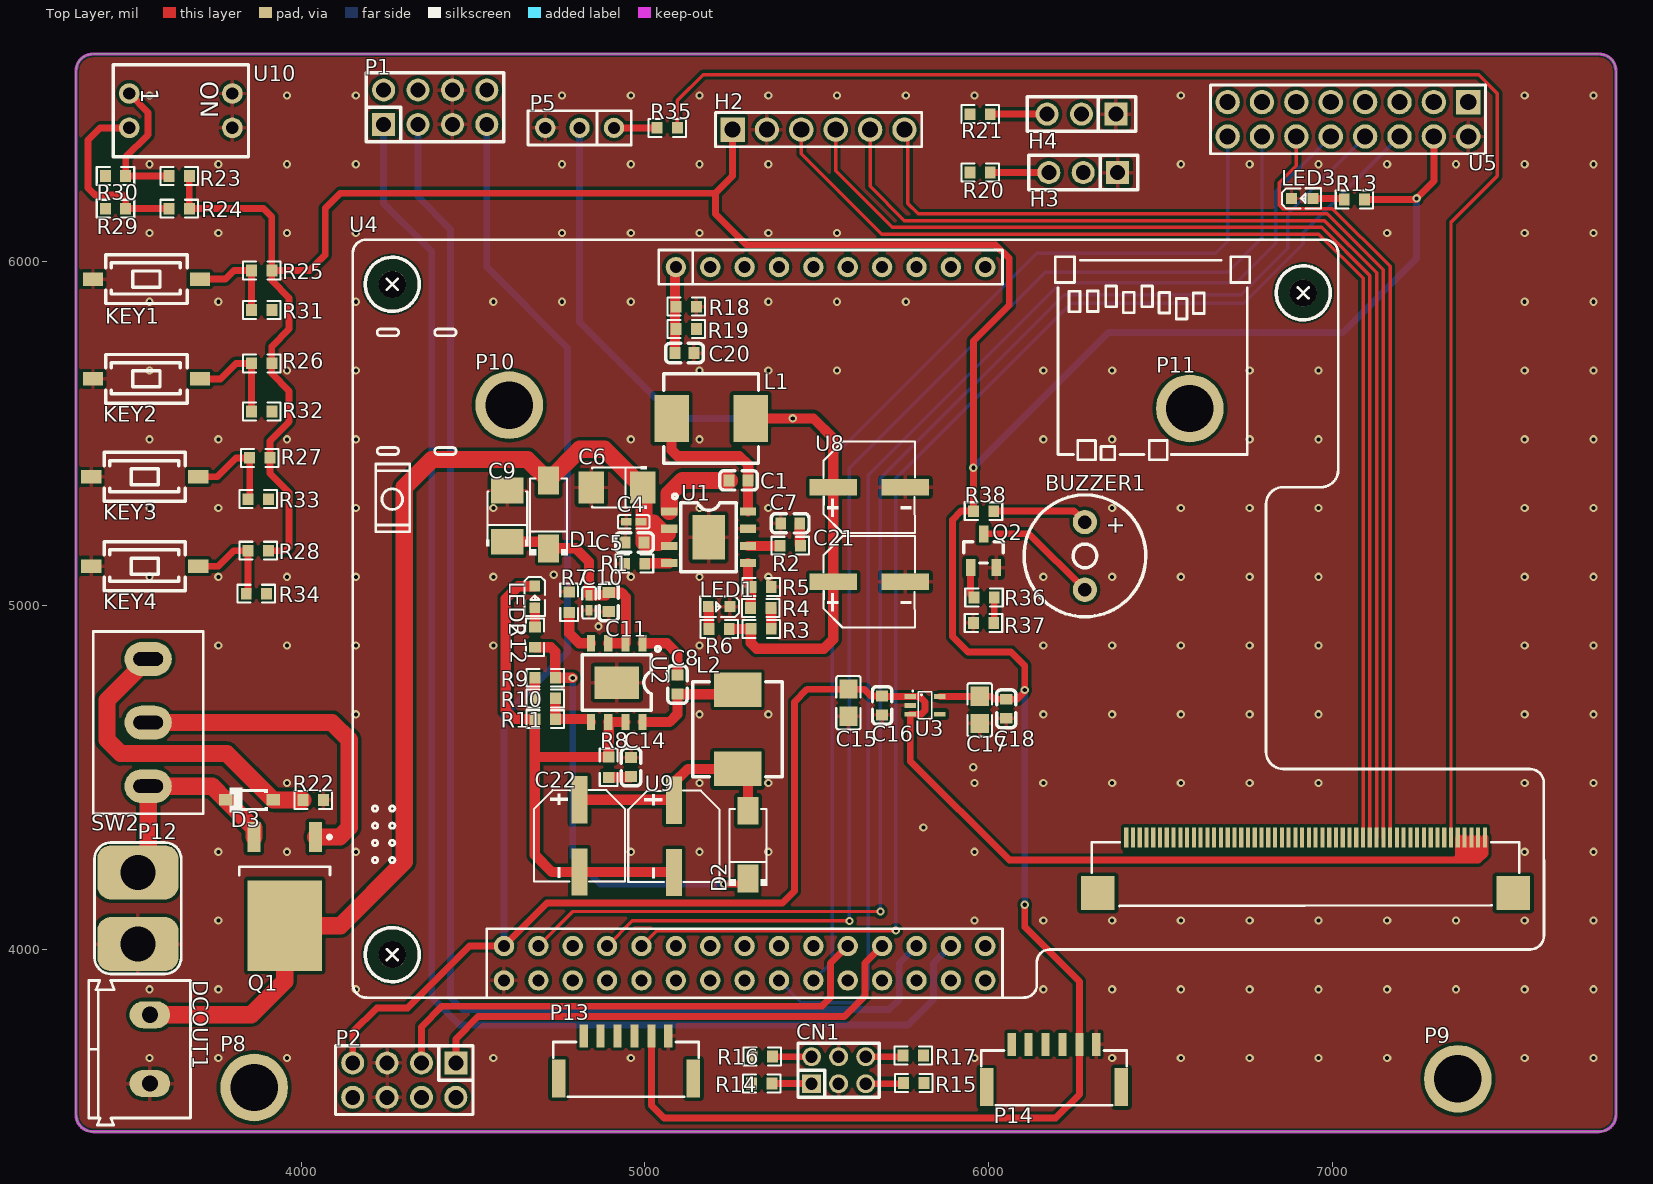
[diagram p0: Top Layer view]
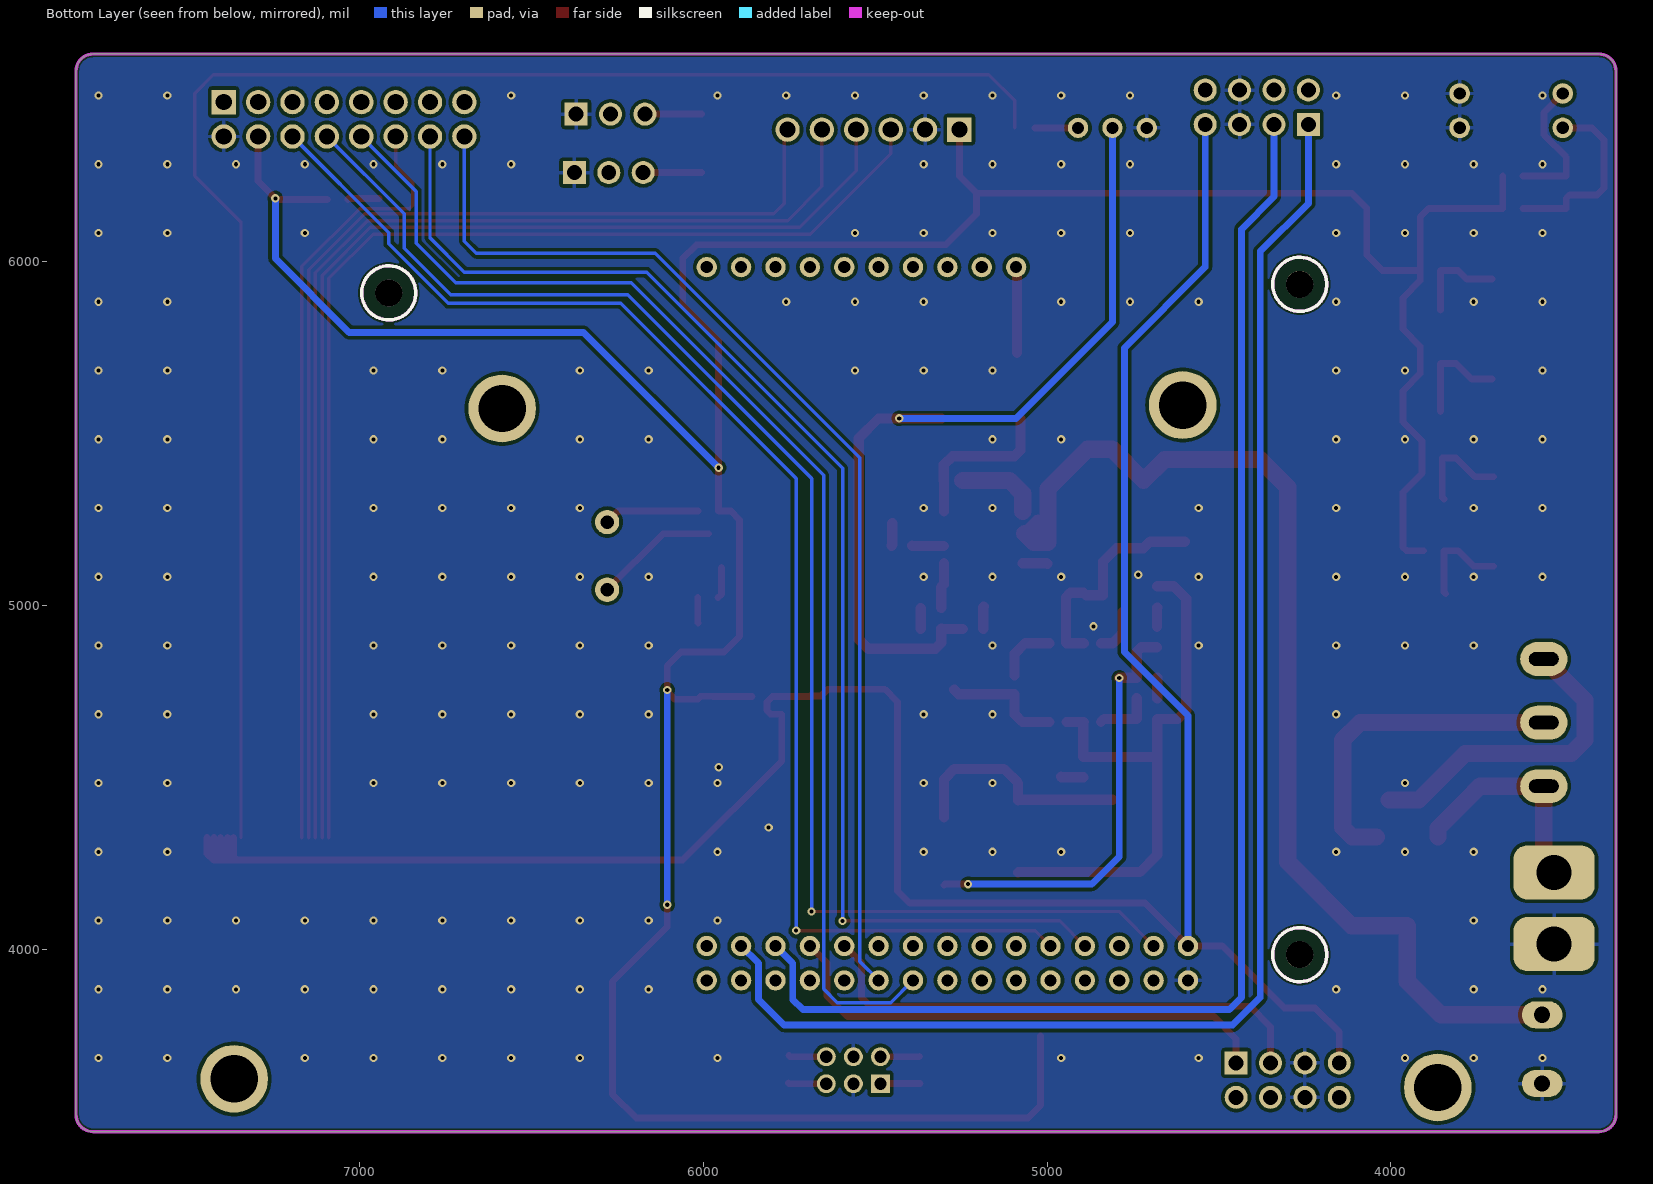
[diagram p1: Bottom Layer view, seen from below]
# Altium PCB MISC62349.pcbdoc
Units mil, origin at the board's own origin, x right, y up, seen from the top; angles counter-clockwise.
Board outline 4479.92 x 3135.04 mil, 2 copper layers (Top Layer, Bottom Layer), stack 62.206 mil thick; 94 components, 95 nets, 352 pads, 194 vias.

## Layer stack, top to bottom
Top Solder Mask Layer: solder mask 0.394, Dk 3.3
Top Layer: signal copper 1.379
Dielectric1: surface 59.449, FR4, Dk 4.5
Bottom Layer: signal copper 1.378
Bottom Solder Mask Layer: solder mask 0.394, Dk 3.3

## Board outline
3395,6605 ccw(c3395,6555) 3345,6555 3345,3519.96 ccw(c3395,3519.96) 3395,3469.96 7774.92,3469.96 ccw(c7774.92,3519.96) 7824.92,3519.96 7824.92,6555 ccw(c7774.92,6555) 7774.92,6605

## Design rules (kind name [scope] priority, off if disabled: settings)
BoardOutlineClearance copperThickness2oz_1 [All] p2 off: genericclearance=7.99 ignorepadtopadclearanceinfootprint=FALSE except(0: Arc-SplitContinuation Track-SplitContinuation SMDPad-SplitContinuation THPad-SplitContinuation Via-SplitContinuation Fill-SplitContinuation Region-SplitContinuation Poly-SplitContinuation Text-SplitContinuation Hole-SplitContinuation; 5.98: Arc-CutoutEdge Track-CutoutEdge SMDPad-CutoutEdge THPad-CutoutEdge Via-CutoutEdge Text-CutoutEdge; 6.9: Hole-OutlineEdge Hole-CutoutEdge; 10: Poly-OutlineEdge Poly-CutoutEdge; 11.81: Arc-OutlineEdge Track-OutlineEdge SMDPad-OutlineEdge THPad-OutlineEdge Via-OutlineEdge Fill-OutlineEdge Region-OutlineEdge Text-OutlineEdge Fill-CutoutEdge Region-CutoutEdge)
BoardOutlineClearance Plane_innerPlane_1 [All] p4 off: genericclearance=4.02 ignorepadtopadclearanceinfootprint=FALSE except(0: Arc-SplitContinuation Track-SplitContinuation SMDPad-SplitContinuation THPad-SplitContinuation Via-SplitContinuation Fill-SplitContinuation Region-SplitContinuation Poly-SplitContinuation Text-SplitContinuation Hole-SplitContinuation; 5.98: Arc-CutoutEdge Track-CutoutEdge SMDPad-CutoutEdge THPad-CutoutEdge Via-CutoutEdge Text-CutoutEdge; 6.9: Hole-OutlineEdge Hole-CutoutEdge; 10: Poly-OutlineEdge Poly-CutoutEdge; 11.81: Arc-OutlineEdge Track-OutlineEdge SMDPad-OutlineEdge THPad-OutlineEdge Via-OutlineEdge Fill-OutlineEdge Region-OutlineEdge Text-OutlineEdge Fill-CutoutEdge Region-CutoutEdge)
BoardOutlineClearance Copper_copperRegion_1 [All] p6 off: genericclearance=4.02 ignorepadtopadclearanceinfootprint=FALSE except(0: Arc-SplitContinuation Track-SplitContinuation SMDPad-SplitContinuation THPad-SplitContinuation Via-SplitContinuation Fill-SplitContinuation Region-SplitContinuation Poly-SplitContinuation Text-SplitContinuation Hole-SplitContinuation; 5.98: Arc-CutoutEdge Track-CutoutEdge SMDPad-CutoutEdge THPad-CutoutEdge Via-CutoutEdge Text-CutoutEdge; 6.9: Hole-OutlineEdge Hole-CutoutEdge; 10: Poly-OutlineEdge Poly-CutoutEdge; 11.81: Arc-OutlineEdge Track-OutlineEdge SMDPad-OutlineEdge THPad-OutlineEdge Via-OutlineEdge Fill-OutlineEdge Region-OutlineEdge Text-OutlineEdge Fill-CutoutEdge Region-CutoutEdge)
BoardOutlineClearance copperThickness1oz_1 [All] p8: genericclearance=4.02 ignorepadtopadclearanceinfootprint=FALSE except(0: Arc-SplitContinuation Track-SplitContinuation SMDPad-SplitContinuation THPad-SplitContinuation Via-SplitContinuation Fill-SplitContinuation Region-SplitContinuation Poly-SplitContinuation Text-SplitContinuation Hole-SplitContinuation; 5.98: Arc-CutoutEdge Track-CutoutEdge SMDPad-CutoutEdge THPad-CutoutEdge Via-CutoutEdge Text-CutoutEdge; 6.9: Hole-OutlineEdge Hole-CutoutEdge; 10: Poly-OutlineEdge Poly-CutoutEdge; 11.81: Arc-OutlineEdge Track-OutlineEdge SMDPad-OutlineEdge THPad-OutlineEdge Via-OutlineEdge Fill-OutlineEdge Region-OutlineEdge Text-OutlineEdge Fill-CutoutEdge Region-CutoutEdge)
Clearance copperThickness2oz [All] p1 off: gap=7.99 ignorepadtopadclearanceinfootprint=FALSE except(5.98: SMDPad-Track SMDPad-SMDPad THPad-Track SMDPad-THPad THPad-THPad Track-Via SMDPad-Via THPad-Via Via-Via Fill-SMDPad Region-SMDPad Fill-THPad Region-THPad Fill-Via Region-Via Fill-Fill Fill-Region Region-Region Arc-Track Arc-SMDPad Arc-THPad Arc-Via Fill-Arc Region-Arc Arc-Arc Text-Track SMDPad-Text Text-THPad Text-Via Fill-Text Region-Text Arc-Text Text-Text; 6.9: Hole-Track Hole-SMDPad Hole-THPad Hole-Via Fill-Hole Region-Hole Hole-Arc Hole-Text; 10: Poly-Track Poly-SMDPad Poly-THPad Poly-Via Poly-Fill Poly-Region Poly-Poly Poly-Arc Poly-Text Poly-Hole; 11.81: Fill-Track Region-Track)
Clearance Plane_innerPlane [All] p3 off: gap=4.02 ignorepadtopadclearanceinfootprint=FALSE except(5.98: SMDPad-Track SMDPad-SMDPad THPad-Track SMDPad-THPad THPad-THPad Track-Via SMDPad-Via THPad-Via Via-Via Fill-SMDPad Region-SMDPad Fill-THPad Region-THPad Fill-Via Region-Via Fill-Fill Fill-Region Region-Region Arc-Track Arc-SMDPad Arc-THPad Arc-Via Fill-Arc Region-Arc Arc-Arc Text-Track SMDPad-Text Text-THPad Text-Via Fill-Text Region-Text Arc-Text Text-Text; 6.9: Hole-Track Hole-SMDPad Hole-THPad Hole-Via Fill-Hole Region-Hole Hole-Arc Hole-Text; 10: Poly-Track Poly-SMDPad Poly-THPad Poly-Via Poly-Fill Poly-Region Poly-Poly Poly-Arc Poly-Text Poly-Hole; 11.81: Fill-Track Region-Track)
Clearance Copper_copperRegion [All] p5 off: gap=4.02 ignorepadtopadclearanceinfootprint=FALSE except(5.98: SMDPad-Track SMDPad-SMDPad THPad-Track SMDPad-THPad THPad-THPad Track-Via SMDPad-Via THPad-Via Via-Via Fill-SMDPad Region-SMDPad Fill-THPad Region-THPad Fill-Via Region-Via Fill-Fill Fill-Region Region-Region Arc-Track Arc-SMDPad Arc-THPad Arc-Via Fill-Arc Region-Arc Arc-Arc Text-Track SMDPad-Text Text-THPad Text-Via Fill-Text Region-Text Arc-Text Text-Text; 6.9: Hole-Track Hole-SMDPad Hole-THPad Hole-Via Fill-Hole Region-Hole Hole-Arc Hole-Text; 10: Poly-Track Poly-SMDPad Poly-THPad Poly-Via Poly-Fill Poly-Region Poly-Poly Poly-Arc Poly-Text Poly-Hole; 11.81: Fill-Track Region-Track)
Clearance copperThickness1oz [All] p7: gap=4.02 ignorepadtopadclearanceinfootprint=FALSE except(5.98: SMDPad-Track SMDPad-SMDPad THPad-Track SMDPad-THPad THPad-THPad Track-Via SMDPad-Via THPad-Via Via-Via Fill-SMDPad Region-SMDPad Fill-THPad Region-THPad Fill-Via Region-Via Fill-Fill Fill-Region Region-Region Arc-Track Arc-SMDPad Arc-THPad Arc-Via Fill-Arc Region-Arc Arc-Arc Text-Track SMDPad-Text Text-THPad Text-Via Fill-Text Region-Text Arc-Text Text-Text; 6.9: Hole-Track Hole-SMDPad Hole-THPad Hole-Via Fill-Hole Region-Hole Hole-Arc Hole-Text; 10: Poly-Track Poly-SMDPad Poly-THPad Poly-Via Poly-Fill Poly-Region Poly-Poly Poly-Arc Poly-Text Poly-Hole; 11.81: Fill-Track Region-Track)
DiffPairsRouting differentialPair [All] p1: maxlimit=6 minlimit=6 mostfreqgap=6 toplayer_minwidth=5 toplayer_prefwidth=10 toplayer_maxwidth=100 toplayer_mingap=6 toplayer_prefgap=6 toplayer_maxgap=6 bottomlayer_minwidth=5 bottomlayer_prefwidth=10 bottomlayer_maxwidth=100 bottomlayer_mingap=6 bottomlayer_prefgap=6 bottomlayer_maxgap=6 maxuncoupledlength=10
HoleToHoleClearance otherClearance [All] p1: gap=11.81 allowstackedmicrovias=TRUE
Length netLength [All] p1: minlimit=0 maxlimit=0
PasteMaskExpansion pasteMaskExpansion [All] p1: expansion=0
PlaneConnect innerPlane [All] p1: planeconnectstyle=Relief reliefexpansion=20 reliefentries=4 reliefconductorwidth=10 reliefairgap=10
PolygonConnect copperRegion [All] p1: connectstyle=Relief reliefconductorwidth=10 reliefentries=4 polygonreliefangle="90 Angle" airgapwidth=10 via.connectstyle=Relief via.reliefconductorwidth=10 via.reliefentries=4 via.polygonreliefangle="90 Angle" via.airgapwidth=10
RoutingVias viaSize [All] p1: holewidth=12.01 width=24.02 viastyle="Through Hole" minholewidth=11.81 minwidth=19.68 maxholewidth=248.03 maxwidth=393.7
SolderMaskExpansion solderMaskExpansion [IsVia] p1: expansion=-1000 istentingtop=TRUE
SolderMaskExpansion solderMaskExpansion [All] p2: expansion=2 istentingtop=FALSE
Width copperThickness2oz_2 [All] p1 off: maxlimit=100 minlimit=8 preferedwidth=10
Width copperThickness1oz_2 [All] p2: maxlimit=100 minlimit=5 preferedwidth=10

## Components (designator, comment, footprint, x,y, rotation, side; value= is the part's Value field where it differs from the comment)
BUZZER1 "BEEP" BUZ-TH_BD9-P50-D0.6-FD 6280,5145 r270 top
C1 "100nF" C0603 5272.64,5364.58 r0 top
C4 "4.7uF" C0402 4967.21,5243.92 r0 top
C5 "100nF" C0603 4969.76,5183.92 r0 top
C6 "100uF" CAP-SMD_L3.5-W2.8-R-RD 4918.66,5343.92 r0 top
C7 "4.7nF" C0603 5422.64,5239.58 r0 top
C8 "100nF" C0603 5094.67,4770.44 r270 top
C9 "100uF" CAP-SMD_L3.5-W2.8-R-RD 4599.67,5260.44 r270 top
C10 "4.7uF" C0402 4837.42,5008.58 r90 top
C11 "100nF" C0603 4894.67,5010.44 r90 top
C14 "4.7nF" C0603 4959.67,4530.56 r270 top
C15 "10uF" C0805 5592.12,4717.82 r90 top
C16 "100nF" C0603 5690,4710 r90 top
C17 "10uF" C0805 5973.94,4697.19 r90 top
C18 "100nF" C0603 6050.87,4700.26 r90 top
C20 "100nF" C0603 5115,5735 r0 top
C21 "47uF" CAP-SMD_BD6.3-L6.6-W6.6-LS7.3-FD 5652.64,5069.58 r0 top
C22 "47uF" CAP-SMD_BD6.3-L6.6-W6.6-LS7.3-FD 4809.67,4330.44 r270 top
CN1 "A2005WV-2x3P" HDR-TH_6P-P2.00-V-M-R2-C3-S2.00 5563.43,3648.78 r0 top
D1 "SS54" SMA_L4.4-W2.8-LS5.4-R-RD 4719.67,5265.44 r90 top
D2 "SS54" SMA_L4.4-W2.8-LS5.4-R-RD 5300,4305 r90 top
D3 "BZT52C16" SOD-123-L 3850,4435 r180 top
DCOUT1 "DCOUT1" "KF/WJ/DG 301-2P-5.0MM" 3560,3710 r90 top
H2 "2.54-1x6P straight pin" HDR-TH_6P-P2.54-V-M-1 5505,6385 r0 top
H3 "" HDR-TH_3P-P2.54-V-M 6275,6260 r180 top
H4 "" HDR-TH_3P-P2.54-V-M 6270,6430 r180 top
KEY1 "Tact switch 3x6x2.5mm" SW-SMD_L6.0-W3.6-LS8.0 3550,5950 r180 top
KEY2 "Tact switch 3x6x2.5mm" SW-SMD_L6.0-W3.6-LS8.0 3550,5660 r180 top
KEY3 "Tact switch 3x6x2.5mm" SW-SMD_L6.0-W3.6-LS8.0 3545,5375 r180 top
KEY4 "Tact switch 3x6x2.5mm" SW-SMD_L6.0-W3.6-LS8.0 3545,5115 r180 top
L1 "4.7uH" IND-SMD_L7.0-W6.6_VCMT063T 5192.64,5544.58 r0 top
L2 "4.7uH" IND-SMD_L7.0-W6.6_VCMT063T 5269.67,4640.44 r270 top
LED1 "LTST-C190KSKT" LED0603-RD 5215.68,4997.5 r180 top
LED2 "LTST-C190KSKT" LED0603-RD 4679.67,5025.44 r270 top
LED3 "LTST-C190KSKT" LED0603-RD 6912.38,6184.58 r0 top
P1 "Straight header 2X4P 2.54mm" HDR-TH_8P-P2.54-V-M-R2-C4-S2.54 4390,6450 r0 top
P2 "Straight header 2X4P 2.54mm" HDR-TH_8P-P2.54-V-M-R2-C4-S2.54 4300,3620 r180 top
P5 "Header-D-M 1x3P" HDR1X3-M 4910,6390 r180 top
P8 "" 定位孔 3863.38,3598.68 r0 top
P9 "" 定位孔 7364.92,3623.68 r0 top
P10 "" 定位孔 4605.36,5583.68 r0 top
P11 "" 定位孔 6585.36,5573.68 r0 top
P12 "XT60_Header" "Wired T-Header ThroughHole" 3525,4120 r0 top
P13 "GH1.25-6P" ECD-GH1.25-6P-SH 4945,3670 r0 top
P14 "GH1.25-6P" ECD-GH1.25-6P-SH 6190,3645 r0 top
Q1 "HY19P03" TO-252AA 3952.25,4198.24 r270 top
Q2 "S8050" SOT-23(SOT-23-3) 5985,5160 r0 top
R1 "200kΩ" R0603 4969.76,5122.5 r0 top
R2 "20kΩ" R0603 5422.64,5174.58 r0 top
R3 "27kΩ" R0603 5337.81,4932.59 r180 top
R4 "27kΩ" R0603 5337.13,4993.16 r0 top
R5 "7.5kΩ" R0603 5337.81,5054.58 r180 top
R6 "10K" R0603 5215.68,4932.5 r0 top
R7 "200kΩ" R0603 4779.67,5010.44 r270 top
R8 "20kΩ" R0603 4894.67,4530.44 r270 top
R9 "51kΩ" R0603 4709.67,4790.44 r0 top
R10 "1.5kΩ" R0603 4709.67,4730.44 r180 top
R11 "7.5kΩ" R0603 4710,4670 r0 top
R12 "4.7kΩ" R0603 4680.17,4908.73 r270 top
R13 "2.7kΩ" R0603 7064.07,6181.76 r180 top
R14 "100Ω" R0603 5340,3610 r0 top
R15 "100Ω" R0603 5782.17,3611.35 r180 top
R16 "100Ω" R0603 5341.71,3688.78 r180 top
R17 "100Ω" R0603 5780.45,3691.35 r0 top
R18 "20kΩ" R0603 5120,5870 r0 top
R19 "200kΩ" R0603 5120,5805 r180 top
R20 "100Ω" R0603 5975,6260 r180 top
R21 "100Ω" R0603 5975,6430 r180 top
R22 "10K" R0603 4035,4435 r180 top
R23 "4.7kΩ" R0603 3645,6250 r180 top
R24 "4.7kΩ" R0603 3645,6155 r180 top
R25 "4.7kΩ" R0603 3885,5975 r180 top
R26 "4.7kΩ" R0603 3885,5705 r180 top
R27 "4.7kΩ" R0603 3880,5430 r180 top
R28 "4.7kΩ" R0603 3875,5160 r180 top
R29 "470Ω" R0603 3460,6155 r180 top
R30 "470Ω" R0603 3460,6250 r180 top
R31 "100Ω" R0603 3885,5860 r0 top
R32 "100Ω" R0603 3885,5565 r0 top
R33 "100Ω" R0603 3875,5310 r0 top
R34 "100Ω" R0603 3870,5035 r0 top
R35 "100Ω" R0603 5065,6390 r180 top
R36 "4.7kΩ" R0603 5986.46,5023.78 r180 top
R37 "1kΩ" R0603 5985,4950 r180 top
R38 "10Ω" R0603 5985,5275 r0 top
SW2 "SS-12D10L9" MTS-10x 3555,4660 r90 top
U1 "SCT2450CQSTER" ESOP-8_L4.9-W3.9-P1.27-LS6.0-BL-EP 5185.56,5198.92 r270 top
U2 "SCT2450CQSTER" ESOP-8_L4.9-W3.9-P1.27-LS6.0-BL-EP 4918.28,4776.23 r180 top
U3 "RT9013-33GU5" SC-70-5_L2.0-W1.3-P0.65-LS2.1-BR 5815,4710 r180 top
U4 "Loongson 2K0300 development board" 龙芯2K0300久久派开发板 4265,3985 r0 top
U5 "2X8PIN2.54" HDR-TH_16P-P2.54-V-M-R2-C8-S2.54 7045,6415 r180 top
U8 "220uF" CAP-SMD_BD6.3-L6.6-W6.6-LS7.2-FD 5652.64,5344.58 r0 top
U9 "220uF" CAP-SMD_BD6.3-L6.6-W6.6-LS7.2-FD 5084.43,4328.94 r270 top
U10 "2-position DIP switch" SW-TH_4P-L9.9-W6.8-P7.62-BL 3650,6440 r270 top

## Footprints (in the part's own frame and the unit in brackets; to place one, negate y for a bottom-side part, rotate by r counter-clockwise, add the part's x,y. Pads: shape width x height; smd on the part's side, far side on the other; paste and mask are expansions set on the pad)
BUZ-TH_BD9-P50-D0.6-FD [mm]
  round 1.8 hole 1: 1(-2.5,0) 2(2.5,0)
  silkscreen extent -4.5,-4.5 4.5,4.5
C0402 [mm]
  rect 0.79x0.54 smd paste-100 mask+0.051: 1(-0.545,0) 2(0.545,0)
  silkscreen extent -1.17,-0.5 1.17,0.5
C0603 [mm]
  rect 0.8x0.9 smd: 1(-0.7,0) 2(0.7,0)
  silkscreen extent -1.39,-0.71 1.39,0.71
C0805 [mm]
  rect 1.41x1.35 smd paste-100 mask+0.051: 1(-1,0) 2(1,0)
  silkscreen extent -1.96,-0.9 1.96,0.9
CAP-SMD_BD6.3-L6.6-W6.6-LS7.2-FD [mm]
  rect 3.5x1.2 smd: 1(-2.67,0) 2(2.67,0)
  silkscreen extent -3.38,-3.38 3.38,3.38
CAP-SMD_BD6.3-L6.6-W6.6-LS7.3-FD [mm]
  rect 3.5x1.2 smd: 1(-2.67,0) 2(2.67,0)
  silkscreen extent -3.38,-3.38 3.38,3.38
CAP-SMD_L3.5-W2.8-R-RD [mm]
  rect 1.9x2.376 smd: 1(1.899,0) 2(-1.899,0)
  silkscreen extent -1.83,-1.55 2.21,1.55
ECD-GH1.25-6P-SH [mm]
  rect 1x2.8 smd: 0(-4.975,-1.15) 0(4.975,-1.15)
  rect 0.6x1.7 smd: 1(3.125,2) 2(1.875,2) 3(0.625,2) 4(-0.625,2) 5(-1.875,2) 6(-3.125,2)
  silkscreen extent -5.38,-2.5 5.38,1.55
ESOP-8_L4.9-W3.9-P1.27-LS6.0-BL-EP [mm]
  rect 0.6x1.2 smd: 1(-1.905,-2.908) 2(-0.635,-2.908) 3(0.635,-2.908) 4(1.905,-2.908) 5(1.905,2.908) 6(0.635,2.908) 7(-0.635,2.908) 8(-1.905,2.908)
  rect 3.3x2.4 smd: 9(0,0)
  silkscreen extent -3.2,-2.67 2.55,2.05
HDR1X3-M [mm]
  round 1.5 hole 0.9: 1(0,0) 2(2.54,0) 3(5.08,0)
  silkscreen extent -1.27,-1.27 6.35,1.27
HDR-TH_3P-P2.54-V-M [mm]
  rect 1.7x1.7 hole 1.1: 1(-2.54,0)
  round 1.7 hole 1.1: 2(0,0) 3(2.54,0)
  silkscreen extent -4.02,-1.27 4.02,1.27
HDR-TH_6P-P2.00-V-M-R2-C3-S2.00 [mm]
  rect 1.4x1.4 hole 0.9 paste+0 mask+0.051: 1(-2,-1)
  round 1.4 hole 0.9 paste+0 mask+0.051: 2(-2,1) 3(0,-1) 4(0,1) 5(2,-1) 6(2,1)
  silkscreen extent -3,-2 3,2
HDR-TH_6P-P2.54-V-M-1 [mm]
  rect 1.8x1.8 hole 1.2: 1(-6.35,0)
  round 1.8 hole 1.2: 2(-3.81,0) 3(-1.27,0) 4(1.27,0) 5(3.81,0) 6(6.35,0)
  silkscreen extent -7.62,-1.27 7.62,1.27
HDR-TH_8P-P2.54-V-M-R2-C4-S2.54 [mm]
  rect 1.7x1.7 hole 1.1: 1(-3.81,-1.27)
  round 1.7 hole 1.1: 2(-3.81,1.27) 3(-1.27,-1.27) 4(-1.27,1.27) 5(1.27,-1.27) 6(1.27,1.27) 7(3.81,-1.27) 8(3.81,1.27)
  silkscreen extent -5.08,-2.54 5.08,2.54
HDR-TH_16P-P2.54-V-M-R2-C8-S2.54 [mm]
  rect 1.8x1.8 hole 1.2 paste+0 mask+0.051: 1(-8.89,-1.27)
  round 1.8 hole 1.2 paste+0 mask+0.051: 2(-8.89,1.27) 3(-6.35,-1.27) 4(-6.35,1.27) 5(-3.81,-1.27) 6(-3.81,1.27) 7(-1.27,-1.27) 8(-1.27,1.27) 9(1.27,-1.27) 10(1.27,1.27) 11(3.81,-1.27) 12(3.81,1.27) 13(6.35,-1.27) 14(6.35,1.27) 15(8.89,-1.27) 16(8.89,1.27)
  silkscreen extent -10.16,-2.54 10.16,2.54
IND-SMD_L7.0-W6.6_VCMT063T [mm]
  rect 2.55x3.5 smd: 1(-2.925,0) 2(2.925,0)
  silkscreen extent -3.5,-3.3 3.5,3.3
"KF/WJ/DG 301-2P-5.0MM" [mm]
  oval 2x3 hole 1.2: 1(2.54,0) 2(-2.54,0)
  silkscreen extent -5.6,-3 5.08,4.53
LED0603-RD [mm]
  rect 0.8x0.8 smd: 1(-0.799,0) 2(0.799,0)
  silkscreen extent -1.49,-0.75 1.39,0.76
MTS-10x [mm]
  oval 2.5x3.5 hole 1 slot 2.2 at 90 deg unplated: 1(-4.7,0) 2(0,0) 3(4.7,0)
  silkscreen extent -6.73,-4.06 6.73,4.06
R0603 [mil]
  rect 31.75x34.02 smd paste-3937.01 mask+2: 1(-29.66,0) 2(29.66,0)
  silkscreen extent -55,-26 55,26
SC-70-5_L2.0-W1.3-P0.65-LS2.1-BR [mm]
  rect 0.85x0.35 smd paste+0 mask+0.05: 1(1.1,-0.65) 2(1.1,0) 3(1.1,0.65) 4(-1.1,0.65) 5(-1.1,-0.65)
  silkscreen extent -0.5,-1.12 0.96,1
SMA_L4.4-W2.8-LS5.4-R-RD [mil]
  rect 81.2x60.59 smd: 1(98.57,0) 2(-98.57,0)
  silkscreen extent -119,-56 104,56
SOD-123-L [mm]
  rect 1x0.85 smd: A(-1.75,0) K(1.75,0)
  silkscreen extent -1.32,-0.9 1.48,0.9
SOT-23(SOT-23-3) [mm]
  rect 0.7x1.25 smd paste+0 mask+0.102: 1(-0.95,-1.25) 2(0.95,-1.25) 3(0,1.25)
  silkscreen extent -1.46,-0.9 1.46,0.65
SW-SMD_L6.0-W3.6-LS8.0 [mm]
  rect 1.5x1 smd: 1(-3.95,0) 2(3.95,0)
  silkscreen extent -3,-1.8 3,1.8
SW-TH_4P-L9.9-W6.8-P7.62-BL [mil]
  round 60 hole 36 paste+0 mask+1.97: 1(-50,-150) 2(50,-150) 3(50,150) 4(-50,150)
  silkscreen extent -134,-197 134,197
TO-252AA [mm]
  rect 6.7x5.5 smd paste+0.102 mask-6.7: 1(3.275,0)
  rect 2.2x0.95 smd paste+0.102 mask-2.2: 2(-3.275,2.28) 3(-3.275,-2.28)
  silkscreen extent -3.4,-3.35 -0.47,3.43
"Wired T-Header ThroughHole" [mm]
  rrect50% 6x4 hole 2.6: 1(0,2.65) 2(0,-2.65)
  silkscreen extent -3.2,-4.85 3.2,4.85
定位孔 [mm]
  round 5 hole 3.5: 1(0,0)
龙芯2K0300久久派开发板 [mm]
  round 2 hole 2 unplated paste+0.102 mask+0: 0(0,0) 0(0,49.53) 0(67.31,48.895)
  round 1.5 hole 0.9: 1(8.255,-1.905) 2(8.255,0.635) 3(10.795,-1.905) 4(10.795,0.635) 5(13.335,-1.905) 6(13.335,0.635) 7(15.875,-1.905) 8(15.875,0.635) 9(18.415,-1.905) 10(18.415,0.635) 11(20.955,-1.905) 12(20.955,0.635) 13(23.495,-1.905) 14(23.495,0.635) 15(26.035,-1.905) 16(26.035,0.635) 17(28.575,-1.905) 18(28.575,0.635) 19(31.115,-1.905) 20(31.115,0.635) 21(33.655,-1.905) 22(33.655,0.635) 23(36.195,-1.905) 24(36.195,0.635) 25(38.735,-1.905) 26(38.735,0.635) 27(41.275,-1.905) 28(41.275,0.635) 29(43.815,-1.905) 30(43.815,0.635) 31(20.955,50.8) 32(23.495,50.8) 33(26.035,50.8) 34(28.575,50.8) 35(31.115,50.8) 36(33.655,50.8) 37(36.195,50.8) 38(38.735,50.8) 39(41.275,50.8) 40(43.815,50.8)
  rect 2.5x2.5 smd: 41(52.13,4.55) 41(82.83,4.55)
  rect 0.305x1.5 smd: 42(80.73,8.65) 43(80.23,8.65) 44(79.73,8.65) 45(79.23,8.65) 46(78.73,8.65) 47(78.23,8.65) 48(77.73,8.65) 49(77.23,8.65) 50(76.73,8.65) 51(76.23,8.65) 52(75.73,8.65) 53(75.23,8.65) 54(74.73,8.65) 55(74.23,8.65) 56(73.73,8.65) 57(73.23,8.65) 58(72.73,8.65) 59(72.23,8.65) 60(71.73,8.65) 61(71.23,8.65) 62(70.73,8.65) 63(70.23,8.65) 64(69.73,8.65) 65(69.23,8.65) 66(68.73,8.65) 67(68.23,8.65) 68(67.73,8.65) 69(67.23,8.65) 70(66.73,8.65) 71(66.23,8.65) 72(65.73,8.65) 73(65.23,8.65) 74(64.73,8.65) 75(64.23,8.65) 76(63.73,8.65) 77(63.23,8.65) 78(62.73,8.65) 79(62.23,8.65) 80(61.73,8.65) 81(61.23,8.65) 82(60.73,8.65) 83(60.23,8.65) 84(59.73,8.65) 85(59.23,8.65) 86(58.73,8.65) 87(58.23,8.65) 88(57.73,8.65) 89(57.23,8.65) 90(56.73,8.65) 91(56.23,8.65) 92(55.73,8.65) 93(55.23,8.65) 94(54.73,8.65) 95(54.23,8.65)
  Board Outline Layer circle w0.254: c0,49.53 r2
  Board Outline Layer circle w0.254: c0,49.53 r2
  Board Outline Layer circle w0.254: c0,0 r2
  Board Outline Layer circle w0.254: c0,0 r2
  Board Outline Layer circle w0.254: c67.31,48.895 r2
  Board Outline Layer circle w0.254: c67.31,48.895 r2
  silkscreen extent -2.91,-3.18 85.09,52.83

## Via types
v1: diameter 24.02, hole 12, Top Layer to Bottom Layer, 194 vias

## Nets (pads, with @x,y where several pads share a name; then routed paths per layer and width w, separated by ;. In a path a pad name is that pad's centre, name@x,y a point inside that pad or via, vN(x,y) a via of type N, cw(c..) or ccw(c..) an arc to the next point about the centre after c; other vN are vias at no path point)
$1N451: C1.1 U1.1 | length 242.1
  Top Layer w50: U1.1 5071.06,5326.06 5109.58,5364.58 C1.1
$1N463: C1.2 L1.1 U1.8 | length 468.4
  Top Layer w30: L1.1 5077.49,5452.51 5095,5435 5275,5435 5300.2,5409.8 C1.2 5300.06,5364.45 U1.8
$1N1022: R1.2 U1.4 | length 72.2
  Top Layer w30: R1.2 5000.84,5123.92 U1.4
$1N1107: C7.2 R2.2 | length 65.9
  Top Layer w30: C7.2 5450.2,5176.68 R2.2
$1N1148: R2.1 U1.6 | length 93.2
  Top Layer w30: U1.6 5392.32,5173.92 R2.1
$1N1224: R3.1 R4.2 | length 60.9
  Top Layer w30: R4.2 5367.47,4992.48 R3.1
$1N1335: R4.1 R5.2 U1.5 | length 134.4
  Top Layer w30: U1.5 5300.06,5062.67 R5.2 5308.15,4993.84 R4.1
$1N1674: LED1.2 R6.1 | length 65.7
  Top Layer w30: LED1.2 5186.02,4995.68 R6.1
$1N1873: C8.1 U2.1 | length 176.3
  Top Layer w30: U2.1 5064.27,4890.73 5094.67,4860.33 C8.1
$1N1882: C8.2 L2.1 U2.8 | length 349.4
  Top Layer w30: U2.8 5071.73,4661.73 5094.67,4684.67 C8.2 5256.95,4742.88 L2.1
$1N1889: C9.1 C10.2 C11.2 D1.2 U2.2 U2.3 | length 660.6
  Top Layer w30: C9.1 4700.85,5185.69 D1.2 4798.13,5166.87 4837.42,5127.58 C10.2 4886.7,5030.04 C11.2 4932,5038 4945,5025 4945,4892.45 U2.2 U2.3
$1N2050: R7.2 U2.4 | length 136.3
  Top Layer w30: R7.2 4779.67,4920.33 4809.27,4890.73 U2.4
$1N2279: C22.2 LED2.1 R8.1 R11.1 U2.6 U2.7 U9.2 | length 1708.1
  Top Layer w30: LED2.1 4631.92,5056.92 4595,5020 4595,4695 4619.56,4670.44 4680.01,4670.44 4680.01,4560.1 ; U2.7 U2.6 4894.67,4660.35 R8.1 4680.01,4560.1 ; U9.2 5082.94,4225.32 C22.2 4729.68,4225.32 4680.01,4274.99 4680.01,4560.1
$1N2284: C22.1 D2.1 L2.2 U9.1 | length 681.6
  Top Layer w30: C22.1 5082.93,4435.56 U9.1 5084.43,4484.43 5125.29,4525.29 L2.2 5299.67,4495.29 D2.1@5299.67,4384.01
$1N2422: C14.2 R8.2 | length 65.9
  Top Layer w30: R8.2 4957.45,4500.78 C14.2
$1N2551: R9.1 R10.2 | length 60
  Top Layer w30: R10.2 R9.1
$1N2627: R10.1 R11.2 U2.5 | length 167.6
  Top Layer w30: R10.1 4739.33,4670.44 4834.58,4670.44 U2.5
$1N2679: D2.2 R9.2 R12.2 | length 1254.9
  Top Layer w20: v1(5230,4190) 5296.54,4190 D2.2@5299.67,4186.87
  Top Layer w30: R12.2 4725.93,4879.07 4739.33,4865.67 R9.2 4789.56,4790.44 v1(4790,4790)
  Bottom Layer w20: v1(4790,4790) 4790,4270 4870,4190 v1(5230,4190)
$1N2807: LED2.2 R12.1 | length 55.8
  Top Layer w30: LED2.2 4680.17,4993.46 R12.1
$1N3286: LED3.2 R13.2 | length 91.7
  Top Layer w20: LED3.2 7031.58,6184.58 R13.2
$1N5845: CN1.1 R14.2 | length 115.3
  Top Layer w20: R14.2 5484.1,3610 CN1.1
$1N5850: R14.1
$1N5855: CN1.5 R15.2 | length 111.1
  Top Layer w20: CN1.5 5750.57,3609.41 R15.2
$1N5861: R15.1
$1N5866: CN1.2 R16.1 | length 113.6
  Top Layer w20: R16.1 5372,3688.15 CN1.2
$1N5872: R16.2
$1N5877: CN1.6 R17.1 | length 109.9
  Top Layer w20: CN1.6 5747.59,3688.15 R17.1
$1N5883: R17.2
$1N6431: H3.3 R20.1 | length 170.3
  Top Layer w20: R20.1 H3.3
$1N6442: H4.3 R21.1 | length 165.3
  Top Layer w20: R21.1 H4.3
$1N6456: R20.2
$1N6461: R21.2
$1N11656: D3.K P12.1 Q1.3 SW2.1 | length 647.2
  Top Layer w50: P12.1 3555,4254.33 SW2.1 3741.14,4474.96 D3.K 3862.48,4353.62 Q1.3
$1N11660: D3.A R22.2 SW2.3 | length 927.6
  Top Layer w50: SW2.3 3435,4725.04 3435,4610 3475,4570 3783.9,4570 D3.A R22.2
$1N12598: R23.2 R30.1 U10.1 | length 415.5
  Top Layer w20: U10.1 3555,6435.01 3555,6370 3489.66,6304.66 R30.1 R23.2
$1N12628: KEY4.1 R28.2 R34.1 | length 290.5
  Top Layer w20: KEY4.1 3760,5115 3805,5160 R28.2 3845.34,5040 R34.1
$1N12656: R24.2 R29.1 U10.2 | length 552.5
  Top Layer w20: U10.2 3414.99,6389.99 3380,6355 3380,6215 3400,6195 3480,6195 3489.66,6185.34 R29.1 R24.2
$1N12706: KEY1.1 R25.2 R31.1 | length 275.2
  Top Layer w20: KEY1.1 3780,5950 3805,5975 R25.2 R31.1
$1N12755: KEY2.1 R26.2 R32.1 | length 308.5
  Top Layer w20: KEY2.1 3765,5660 3810,5705 R26.2 R32.1
$1N12808: KEY3.1 R27.2 R33.1 | length 294.7
  Top Layer w20: KEY3.1 3755,5375 3810,5430 R27.2 3850.34,5315 R33.1
$1N12981: Q1.2 SW2.2 | length 970.2
  Top Layer w50: SW2.2 4090,4660 4140,4610 4140,4355 4112.18,4327.18 Q1.2
$1N13231: P5.1 R35.2 | length 125.3
  Top Layer w20: P5.1 R35.2
$1N16231: BUZZER1.1 R38.2 | length 278.4
  Top Layer w20: R38.2 6248.43,5275 BUZZER1.1
$1N16240: BUZZER1.2 Q2.3 | length 362.4
  Top Layer w20: Q2.3 6117.37,5209.2 BUZZER1.2
$1N16252: R36.1 R37.1 | length 74.4
  Top Layer w20: R37.1 6016.12,4951.46 R36.1
$1N16259: Q2.1 R36.2 | length 90.8
  Top Layer w20: Q2.1 5947.6,5032.97 R36.2
ADC7: C20.1 R18.1 R19.2 U4.31 | length 251.1
  Top Layer w30: C20.1 5087.44,5982.44 U4.31
GND: C4.1 C5.1 C6.2 C7.1 C9.2 C10.1 C11.1 C14.1 C15.1 C16.1 C17.1 C18.1 C20.2 C21.2 CN1.3 CN1.4 DCOUT1.2 H2.2 H3.1 H4.1 KEY1.2 KEY2.2 KEY3.2 KEY4.2 LED1.1 LED3.1 P1.5 P1.6 P2.5 P2.6 P5.3 P12.2 P13.1 P14.1 Q2.2 R1.1 R5.1 R7.1 R18.2 R22.1 R37.2 U1.7 U1.9 U2.9 U3.2 U4.1 U5.2 U8.2 U10.3 U10.4
  other v1: 3559.1,3684.06 3759.1,3684.06 3959.1,3684.06 4559.1,3684.06 4959.1,3684.06 5959.1,3684.06 6359.1,3684.06 6559.1,3684.06 6759.1,3684.06 6959.1,3684.06 7159.1,3684.06 7559.1,3684.06 7759.1,3684.06 3559.1,3884.06 3759.1,3884.06 4159.1,3884.06 6159.1,3884.06 6359.1,3884.06 6559.1,3884.06 6759.1,3884.06 6959.1,3884.06 7159.1,3884.06 7359.1,3884.06 7559.1,3884.06 7759.1,3884.06 3759.1,4084.06 5959.1,4084.06 6159.1,4084.06 6359.1,4084.06 6559.1,4084.06 6759.1,4084.06 6959.1,4084.06 7159.1,4084.06 7359.1,4084.06 7559.1,4084.06 7759.1,4084.06 3759.1,4284.06 3959.1,4284.06 4159.1,4284.06 4959.1,4284.06 5159.1,4284.06 5359.1,4284.06 5959.1,4284.06 7559.1,4284.06 7759.1,4284.06 5810,4355 3959.1,4484.06 5159.1,4484.06 5359.1,4484.06 5959.1,4484.06 6159.1,4484.06 6359.1,4484.06 6559.1,4484.06 6759.1,4484.06 6959.1,4484.06 7559.1,4484.06 7759.1,4484.06 5955,4530 4159.1,4684.06 5159.1,4684.06 5359.1,4684.06 6159.1,4684.06 6359.1,4684.06 6559.1,4684.06 6759.1,4684.06 6959.1,4684.06 7559.1,4684.06 7759.1,4684.06 3759.1,4884.06 3959.1,4884.06 4159.1,4884.06 4559.1,4884.06 5159.1,4884.06 6159.1,4884.06 6359.1,4884.06 6559.1,4884.06 6759.1,4884.06 6959.1,4884.06 7559.1,4884.06 7759.1,4884.06 4865,4940 3559.1,5084.06 3759.1,5084.06 3959.1,5084.06 4159.1,5084.06 4559.1,5084.06 4959.1,5084.06 5159.1,5084.06 5359.1,5084.06 6159.1,5084.06 6359.1,5084.06 6559.1,5084.06 6759.1,5084.06 6959.1,5084.06 7559.1,5084.06 7759.1,5084.06 4735,5090 3559.1,5284.06 3759.1,5284.06 4159.1,5284.06 4559.1,5284.06 5159.1,5284.06 5359.1,5284.06 6359.1,5284.06 6559.1,5284.06 6759.1,5284.06 6959.1,5284.06 7559.1,5284.06 7759.1,5284.06 3559.1,5484.06 3759.1,5484.06 3959.1,5484.06 4159.1,5484.06 4959.1,5484.06 5159.1,5484.06 6159.1,5484.06 6359.1,5484.06 6759.1,5484.06 6959.1,5484.06 7559.1,5484.06 7759.1,5484.06 3559.1,5684.06 3959.1,5684.06 4159.1,5684.06 5159.1,5684.06 5359.1,5684.06 5559.1,5684.06 6159.1,5684.06 6359.1,5684.06 6759.1,5684.06 6959.1,5684.06 7559.1,5684.06 7759.1,5684.06 3559.1,5884.06 3759.1,5884.06 4159.1,5884.06 4559.1,5884.06 4759.1,5884.06 4959.1,5884.06 5359.1,5884.06 5559.1,5884.06 5759.1,5884.06 7559.1,5884.06 7759.1,5884.06 3559.1,6084.06 3759.1,6084.06 3959.1,6084.06 4159.1,6084.06 4759.1,6084.06 4959.1,6084.06 5159.1,6084.06 5359.1,6084.06 5559.1,6084.06 7159.1,6084.06 7559.1,6084.06 7759.1,6084.06 3559.1,6284.06 3759.1,6284.06 3959.1,6284.06 4159.1,6284.06 4759.1,6284.06 4959.1,6284.06 5159.1,6284.06 5359.1,6284.06 6559.1,6284.06 6759.1,6284.06 6959.1,6284.06 7159.1,6284.06 7359.1,6284.06 7559.1,6284.06 7759.1,6284.06 3559.1,6484.06 3959.1,6484.06 4159.1,6484.06 4759.1,6484.06 4959.1,6484.06 5159.1,6484.06 5359.1,6484.06 5559.1,6484.06 5759.1,6484.06 5959.1,6484.06 6559.1,6484.06 7559.1,6484.06 7759.1,6484.06
GPIO012: U4.71
GPIO013: U4.70
GPIO13: R34.2
GPIO014: U4.69
GPIO14: R33.2
GPIO015: U4.68
GPIO15: R32.2
GPIO016: U4.67
GPIO16: R31.2
GPIO020: U4.62
GPIO20: R30.2
GPIO021: U4.61
GPIO21: R29.2
GPIO022: H2.3 U4.60 | length 3481
  Top Layer w10: H2.3 5455,6315.11 5689.16,6080.94 6960.54,6080.94 7089.01,5952.47 U4.60
GPIO023: H2.4 U4.59 | length 3434.8
  Top Layer w10: H2.4 5555,6265 5719.37,6100.63 6968.69,6100.63 7108.7,5960.63 U4.59
GPIO024: H2.5 U4.58 | length 3385.7
  Top Layer w10: H2.5 5655,6220 5754.69,6120.31 6976.85,6120.31 7128.38,5968.78 U4.58
GPIO025: H2.6 U4.57 | length 3333.6
  Top Layer w10: H2.6 5765,6375 5765,6170 5795,6140 6985,6140 7148.07,5976.93 U4.57
GPIO026: U4.56 U5.12 | length 2278.8
  Top Layer w10: U5.12 6895,6280 6845,6230 6845,6165 6855,6155 7000,6155 7167.75,5987.25 U4.56
GPIO040: P1.3 U4.26 | length 4087
  Bottom Layer w20: P1.3 4340,6190 4435,6095 4435,3860 4470,3825 5710,3825 5740,3855 5740,3960 U4.26
GPIO041: P1.1 U4.28 | length 4297.9
  Bottom Layer w20: P1.1 4240,6170 4380,6030 4380,3860 4460,3780 5765,3780 5840,3855 5840,3960 U4.28
GPIO042: P2.3 U4.22 | length 1500.9
  Top Layer w20: P2.3 4350,3775 4410,3835 5515,3835 5540,3860 5540,3960 U4.22
GPIO043: P2.1 U4.24 | length 1477.5
  Top Layer w20: P2.1 4450,3740 4515,3805 5580,3805 5640,3865 5640,3960 U4.24
GPIO50: P14.4
GPIO050: U4.15
GPIO51: P13.4
GPIO051: U4.13
GPIO060: U4.10 U5.6 | length 3969.5
  Top Layer w10: U4.10 5035,4055 v1(5730,4055)
  Bottom Layer w10: v1(5730,4055) 5730,5370 6240,5880 6741.96,5880 6915,6053.04 6915,6085 U5.6
GPIO062: U4.4 U5.8 | length 4176.8
  Top Layer w10: U4.4 4790.57,4110.57 v1(5685,4110.57)
  Bottom Layer w10: v1(5685,4110.57) 5685,5370 6220,5905 6735,5905 6870,6040 6870,6140 U5.8
GPIO063: U4.8 U5.14 | length 3824.8
  Top Layer w10: U4.8 4962.99,4082.99 v1(5595,4082.99)
  Bottom Layer w10: v1(5595,4082.99) 5595,5400 6165,5970 6695,5970 6795,6070 U5.14
GPIO64: P13.3
GPIO064: U4.9
GPIO065: U4.5
GPIO066: U4.3
GPIO67: P14.3
GPIO067: U4.7
GPIO072: U4.21
GPIO073: U4.23
GPIO074: U4.17 U5.10 | length 3639.8
  Bottom Layer w10: U4.17 5455,3845 5610,3845 5650,3885 5650,3892.71 5649.49,3893.22 5649.49,4026.78 5650,4027.29 5650,5380 6210,5940 6720,5940 6835,6055 6835,6205 U5.10
GPIO075: U4.19 U5.16 | length 3259.2
  Bottom Layer w10: U4.19 5545,3965 5545,3990.64 5544.49,3991.15 5544.49,4028.85 5545,4029.36 5545,5430 6140,6025 6660,6025 6695,6060 U5.16
GPIO086: R35.1 U4.47 | length 4739.4
  Top Layer w10: R35.1 5094.66,6469.66 5170,6545 7425,6545 7480,6490 7480,6250 7344.92,6114.92 U4.47
GPIO088: U4.27
GPIO089: U4.25
VCC: R19.1
VCC3V3: C17.2 C18.2 H2.1 P13.2 P14.2 R13.1 R23.1 R24.1 R25.1 R26.1 R27.1 R28.1 R38.1 U3.5 U5.4 | length 10687.8
  Top Layer w20: R23.1 R24.1 3890,6155 3914.66,6130.34 R25.1 ; R28.1 3955,5160 3965,5170 3965,5330 3909.66,5385.34 R27.1 3909.66,5479.66 3965,5535 3965,5625 3914.66,5675.34 R26.1 3914.66,5754.66 3965,5805 3965,5895 3914.66,5945.34 R25.1 ; P13.2 5018.82,3546.18 5055,3510 6195,3510 6263.82,3578.82 P14.2 6263.82,3906.18 6105,4065 v1(6105,4130) ; H2.1 5255,6250 5205,6200 ; U3.5 5972.97,4735.59 C17.2 6008.44,4736.56 6017.18,4727.82 C18.2 6082.82,4727.82 6105,4750 6105,4825 6065,4865 5940,4865 5895,4910 5895,5250 5920,5275 R38.1 v1(5955.34,5401.49) 5955.34,5770.34 6060,5875 6060,6010 6020,6050 5295,6050 5205,6140 5205,6200 ; R13.1 7241.76,6181.76 7295,6235 U5.4 ; R25.1 4025,5975 4070,6020 4070,6155 4115,6200 5205,6200
  Bottom Layer w20: v1(5955.34,5401.49) 6348.85,5795 7030,5795 7245,6010 v1(7245,6185) ; v1(6105,4130) v1(6105,4755)
VCC5V: C15.2 C16.2 P1.7 P2.7 U3.1 U3.3 U4.2 U4.42 U4.43 U4.44 U4.45 U4.46 | length 7413.9
  Top Layer w20: P2.7 4150,3760 4220,3830 4310,3830 4490,4010 U4.2 4715,4135 5400,4135 5435,4170 5435,4720 5472.19,4757.19 C15.2 5637.81,4757.19 5657.44,4737.56 C16.2 5691.97,4735.59 U3.1 5799.41,4735.59 5815,4720 5815,4695 5804.41,4684.41 U3.3 5771.69,4548.31 6060,4260 7356.79,4260 ; U4.46@7366.9,4325.55 7366.9,4270.11 7356.79,4260 ; U4.45 7384.29,4275.58 7368.71,4260 ; U4.44 7403.97,4283.12 7380.85,4260 ; U4.43 7423.66,4277.39 7406.26,4260 ; U4.42 7443.34,4278.34 7425,4260 7406.26,4260 ; 7356.79,4260 7368.71,4260 ; 7368.71,4260 7380.85,4260 ; 7380.85,4260 7406.26,4260
  Bottom Layer w20: P1.7 4540,5985 4775,5750 4775,4865 4590,4680 U4.2
VCCBAT: C4.2 C5.2 C6.1 D1.1 DCOUT1.1 Q1.1 U1.2 U1.3 | length 3237.8
  Top Layer w50: DCOUT1.1 3855,3810 3952.25,3907.25 Q1.1 4114.31,4069.31 4300,4255 4300,5345 4380,5425 4658.68,5425 D1.1 4810.65,5455 4882.33,5455 C6.1 4997.32,5340.01 C5.2 5038.92,5183.92 5065,5210 5055,5210 5024.64,5240.36
VCCSERVO: C21.1 L1.2 P5.2 R3.2 R6.2 U8.1 | length 2510.6
  Top Layer w30: R6.2 5308.06,4932.5 R3.2 5308.15,4891.85 5325,4875 5520,4875 5547.52,4902.52 C21.1 U8.1 5547.52,5487.48 5490.42,5544.58 L1.2
  Bottom Layer w20: P5.2 4810,5825 5090,5545 v1(5430,5545)
pads on no net: H3.2 H4.2 P1.2 P1.4 P1.8 P2.2 P2.4 P2.8 P8.1 P9.1 P10.1 P11.1 P13.0 P13.5 P13.6 P14.0 P14.5 P14.6 U3.4 U4.0 U4.6 U4.11 U4.12 U4.14 U4.16 U4.18 U4.20 U4.29 U4.30 U4.32 U4.33 U4.34 U4.35 U4.36 U4.37 U4.38 U4.39 U4.40 U4.41 U4.48 U4.49 U4.50 U4.51 U4.52 U4.53 U4.54 U4.55 U4.63 U4.64 U4.65 U4.66 U4.72 U4.73 U4.74 U4.75 U4.76 U4.77 U4.78 U4.79 U4.80 U4.81 U4.82 U4.83 U4.84 U4.85 U4.86 U4.87 U4.88 U4.89 U4.90 U4.91 U4.92 U4.93 U4.94 U4.95 U5.1 U5.3 U5.5 U5.7 U5.9 U5.11 U5.13 U5.15

## Polygon pours and split planes (outlines as drawn)
GND on Top Layer (solid, remove dead copper, pour order 0): 3000,6790 3000,3000 8070,3000 8070,6790
GND on Bottom Layer (solid, remove dead copper, pour order 2): 3055,6835 3055,3240 8100,3240 8100,6835

## Keep-outs
Board Outline Layer:
  the board outline again, w10